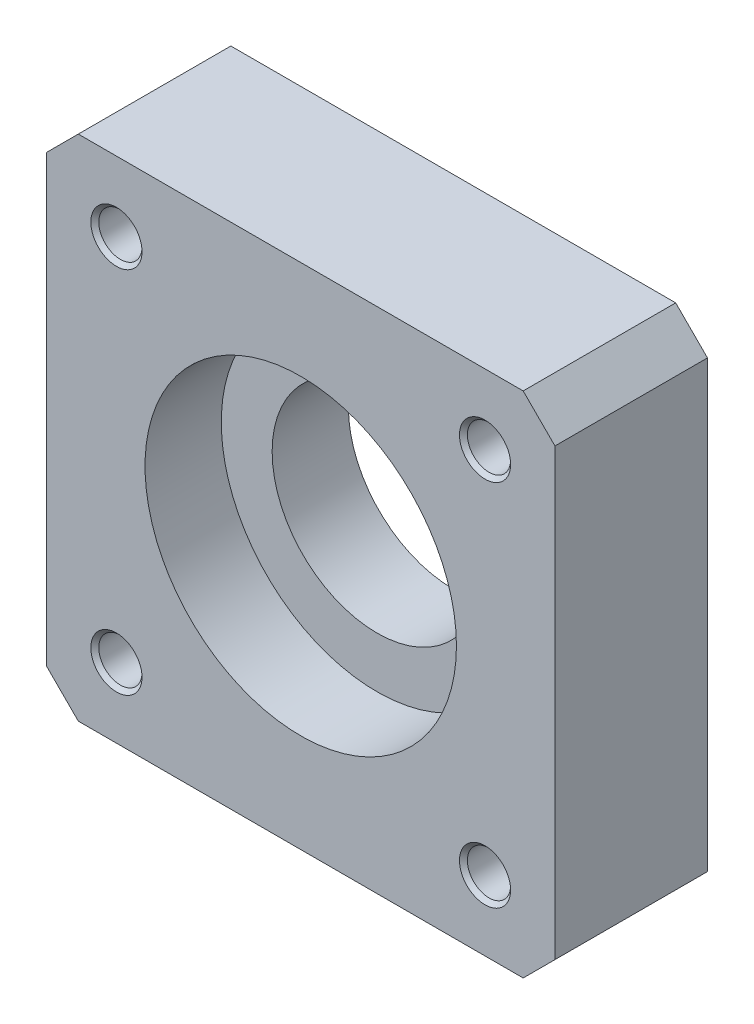
SolidWorks part; units mm, degrees
material "Q235-A"
ref_plane "Front Plane" through (0, 0, 0) normal (0, 0, 1) x (1, 0, 0)
ref_plane "Top Plane" through (0, 0, 0) normal (0, 1, 0) x (1, 0, 0)
ref_plane "Right Plane" through (0, 0, 0) normal (1, 0, 0) x (0, 0, -1)
sketch "Sketch1" plane through (0, 0, 0) normal (0, 0, 1) x (1, 0, 0)
  line L1 (-52.5688, 58.6182) -> (27.4312, 58.6182)
  line L2 (-52.5688, 58.6182) -> (-52.5688, -21.3818)
  line L3 (-52.5688, -21.3818) -> (27.4312, -21.3818)
  line L4 (27.4312, 58.6182) -> (27.4312, -21.3818)
  dimension "D1" = 80
  dimension "D2" = 80
extrude "Boss-Extrude1" add sketch "Sketch1" along normal blind 24
sketch "Sketch2" plane through (0, 0, 24) normal (0, 0, 1) x (1, 0, 0)
  line L0 (27.4312, -21.3818) -> (27.4312, 58.6182) construction
  line L1 (-41.5688, -10.3818) -> (16.4312, -10.3818)
  line L2 (-41.5688, -10.3818) -> (-41.5688, 47.6182)
  line L3 (-41.5688, 47.6182) -> (16.4312, 47.6182)
  line L4 (16.4312, -10.3818) -> (16.4312, 47.6182)
  line L5 (-41.5688, -10.3818) -> (16.4312, 47.6182) construction
  line L6 (-41.5688, 47.6182) -> (16.4312, -10.3818) construction
  line L7 (27.4312, 58.6182) -> (-52.5688, 58.6182) construction
  circle A0 centre (-12.5688, 18.6182) radius 3.699
  dimension "D1" = 58
  dimension "D2" = 58
  dimension "D3" = 11
  dimension "D4" = 11
hole_wizard "Hole1" positions "Sketch3" profile "Sketch4" legacy end condition through all
sketch "Sketch3" plane through (0, 0, 24) normal (0, 0, 1) x (1, 0, 0)
  point P0 (-12.5688, 18.6182)
sketch "Sketch4" plane through (-12.5688, 18.6182, 24) normal (1, 0, 0) x (0, -1, 0)
  line L0 (0, 0) -> (0, 24)
  line L1 (0, 24) -> (16.5, 24)
  line L2 (16.5, 24) -> (16.5, 12)
  line L3 (16.5, 12) -> (24.5, 12)
  line L4 (24.5, 12) -> (24.5, 0)
  line L5 (24.5, 0) -> (0, 0)
  line L6 (0, 110) -> (0, -10) construction
  dimension "直径" = 33
  dimension "深度" = 24
  dimension "柱坑直径" = 49
  dimension "柱坑深度" = 12
hole_wizard "M8 Tapped Hole1" positions "Sketch5" profile "Sketch6" tap size "M8" standard "GB" end condition through all
sketch "Sketch5" plane through (0, 0, 24) normal (0, 0, 1) x (1, 0, 0)
  point P0 (-41.5688, 47.6182)
  point P3 (16.4312, 47.6182)
  point P6 (16.4312, -10.3818)
  point P9 (-41.5688, -10.3818)
sketch "Sketch6" plane through (-41.5688, 47.6182, 24) normal (1, 0, 0) x (0, -1, 0)
  line L0 (0, 0) -> (0, 24)
  line L1 (0, 24) -> (3.4, 24)
  line L2 (3.4, 24) -> (3.4, 0.625)
  line L3 (3.4, 0.625) -> (4.025, 0)
  line L5 (4.025, 0) -> (0, 0)
  line L6 (-3.4, 0.625) -> (-4.025, 0) construction
  line L11 (0, -6.35) -> (0, 107.95) construction
  dimension "通孔螺纹孔钻头直径" = 6.8
  dimension "通孔螺纹孔钻头深度" = 24
  dimension "近端锥形沉头孔直径" = 8.05
  dimension "近端锥形沉头孔角度" = 90
cosmetic thread "Cosmetic thread 1" parameters "D2"=8
cosmetic thread "Cosmetic thread 2" parameters "D2"=8
cosmetic thread "Cosmetic thread 3" parameters "D2"=8
cosmetic thread "Cosmetic thread 4" parameters "D2"=8
chamfer "Chamfer1" distance 5 angle 45 4 edges at (27.4312, 58.6182, 12) (27.4312, -21.3818, 12) (-52.5688, -21.3818, 12) (-52.5688, 58.6182, 12)
